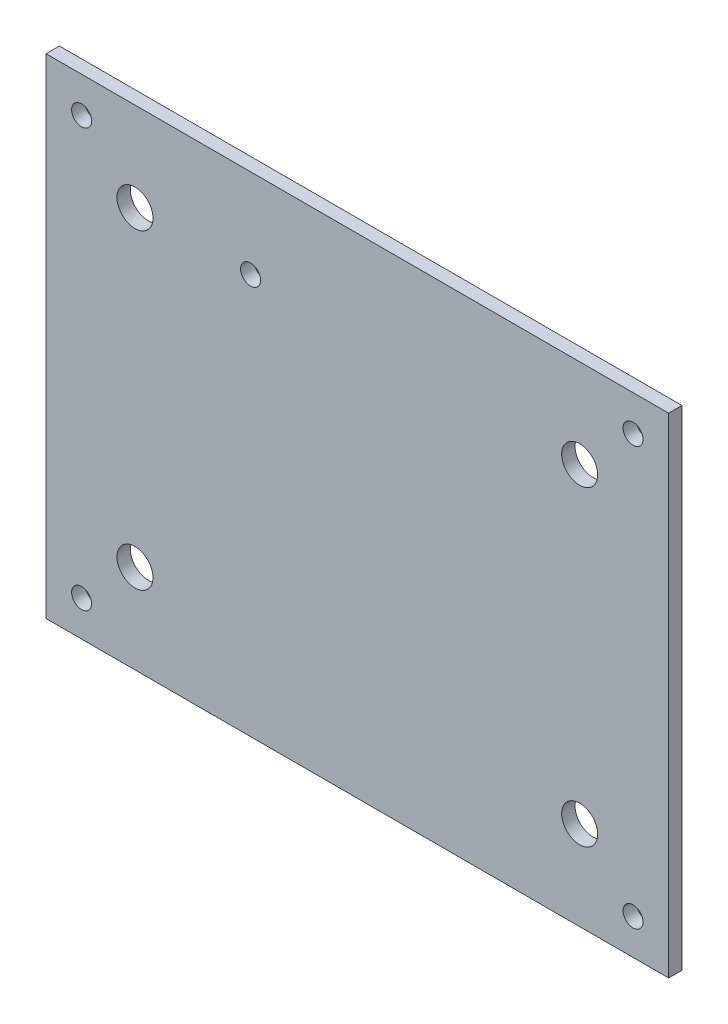
from build123d import *

# Parameters (mm, degrees)
SKETCH_1_W      = 140
SKETCH_1_H      = 110
SKETCH_1_R      = 2.25
SKETCH_1_R_2    = 4.05
EXTRUDE_1_DEPTH = 1.5


with BuildPart() as part:
    # 草图1 → 凸台-拉伸1 (new, symmetric)
    with BuildSketch(Plane.XY):
        Rectangle(SKETCH_1_W, SKETCH_1_H)
        with Locations((-62, -47)):
            Circle(SKETCH_1_R, mode=Mode.SUBTRACT)
        with Locations((-62, 47)):
            Circle(SKETCH_1_R, mode=Mode.SUBTRACT)
        with Locations((62, -47)):
            Circle(SKETCH_1_R, mode=Mode.SUBTRACT)
        with Locations((62, 47)):
            Circle(SKETCH_1_R, mode=Mode.SUBTRACT)
        with Locations((-50, -35)):
            Circle(SKETCH_1_R_2, mode=Mode.SUBTRACT)
        with Locations((-50, 35)):
            Circle(SKETCH_1_R_2, mode=Mode.SUBTRACT)
        with Locations((50, -35)):
            Circle(SKETCH_1_R_2, mode=Mode.SUBTRACT)
        with Locations((50, 35)):
            Circle(SKETCH_1_R_2, mode=Mode.SUBTRACT)
        with Locations((-24, 35)):
            Circle(SKETCH_1_R, mode=Mode.SUBTRACT)
    extrude(amount=EXTRUDE_1_DEPTH, both=True)


solid = part.part
